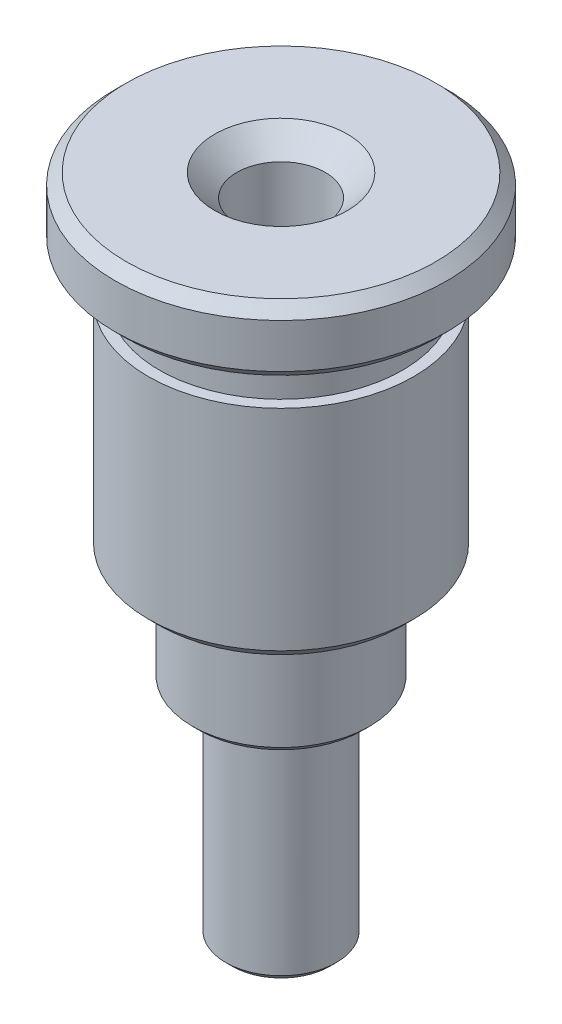
SolidWorks part; units mm, degrees
ref_plane "前视基准面" through (0, 0, 0) normal (0, 0, 1) x (1, 0, 0)
ref_plane "上视基准面" through (0, 0, 0) normal (0, 1, 0) x (1, 0, 0)
ref_plane "右视基准面" through (0, 0, 0) normal (1, 0, 0) x (0, 0, -1)
sketch "草图1" plane through (0, 0, 0) normal (0, 1, 0) x (1, 0, 0)
  circle A0 centre (0, 0) radius 6
  dimension "D1" = 12
extrude "凸台-拉伸1" add sketch "草图1" against normal blind 15
sketch "草图2" plane through (0, -15, 0) normal (0, -1, 0) x (1, 0, 0)
  circle A0 centre (0, 0) radius 2.5
  dimension "D1" = 5
extrude "凸台-拉伸2" add sketch "草图2" along normal blind 15
sketch "草图3" plane through (0, 0, 0) normal (0, 1, 0) x (1, 0, 0)
  circle A0 centre (0, 0) radius 2
  dimension "D1" = 4
extrude "切除-拉伸1" cut sketch "草图3" against normal through all
chamfer "倒角1" [suppressed] distance 1 angle 60
chamfer "倒角2" distance 0.5 angle 45 1 edges at (0, -15, 6)
sketch "草图4" plane through (0, 0, 0) normal (0, 0, 1) x (1, 0, 0)
  line L0 (-6, 0) -> (-6, -14.5) construction
  line L1 (25.8442, 21.4132) -> (5.5, 21.4132)
  line L2 (25.8442, 21.4132) -> (25.8442, -18.6855)
  line L3 (25.8442, -18.6855) -> (5.5, -18.6855)
  line L4 (5.5, 21.4132) -> (5.5, -18.6855)
  line L5 (25.8442, 21.4132) -> (5.5, -18.6855) construction
  line L6 (25.8442, -18.6855) -> (5.5, 21.4132) construction
  line L7 (-25.6968, 35.6394) -> (-5.5, 35.6394)
  line L8 (-25.6968, 35.6394) -> (-25.6968, -22.0025)
  line L9 (-25.6968, -22.0025) -> (-5.5, -22.0025)
  line L10 (-5.5, 35.6394) -> (-5.5, -22.0025)
  line L11 (-25.6968, 35.6394) -> (-5.5, -22.0025) construction
  line L12 (-25.6968, -22.0025) -> (-5.5, 35.6394) construction
  line L13 (6, -14.5) -> (6, 0) construction
  point P0 (15.6721, 1.3638)
  point P5 (-15.5984, 6.8184)
  dimension "D1" = 0.5
  dimension "D2" = 0.5
extrude "切除-拉伸2" [suppressed] cut sketch "草图4" against normal mid plane 20
sketch "草图6" plane through (0, 0, 0) normal (0, 1, 0) x (1, 0, 0)
  circle A0 centre (0, 0) radius 7.5
  circle A1 centre (0, 0) radius 6
  dimension "D1" = 12
  dimension "D2" = 15
extrude "凸台-拉伸3" add sketch "草图6" against normal blind 3
chamfer "倒角3" distance 1 angle 45 1 edges at (0, 0, 2)
chamfer "倒角4" distance 0.5 angle 45 2 edges at (0, -3, 7.5) (0, 0, 7.5)
sketch "草图7" plane through (0, -15, 0) normal (0, -1, 0) x (1, 0, 0)
  circle A0 centre (0, 0) radius 4
  circle A1 centre (0, 0) radius 2.5
  dimension "D1" = 5
  dimension "D2" = 8
extrude "凸台-拉伸4" add sketch "草图7" along normal blind 5
chamfer "倒角5" distance 0.3 angle 45 1 edges at (0, -20, -4)
chamfer "倒角6" distance 0.3 angle 45 1 edges at (0, -30, -2.5)
sketch "草图8" plane through (0, 0, 0) normal (0, 0, 1) x (1, 0, 0)
  line L0 (-6, -3) -> (-6, -14.5) construction
  line L1 (-8.8677, -3) -> (-5.5, -3)
  line L2 (-8.8677, -3) -> (-8.8677, -5)
  line L3 (-8.8677, -5) -> (-5.5, -5)
  line L4 (-5.5, -3) -> (-5.5, -5)
  line L5 (-8.8677, -3) -> (-5.5, -5) construction
  line L6 (-8.8677, -5) -> (-5.5, -3) construction
  line L7 (-7, -3) -> (7, -3) construction
  point P0 (-7.1839, -4)
  dimension "D1" = 2
  dimension "D2" = 0.5
revolve "切除-旋转1" cut sketch "草图8" angle 360 about axis through (0, -15, 0) along (0, 1, 0)
